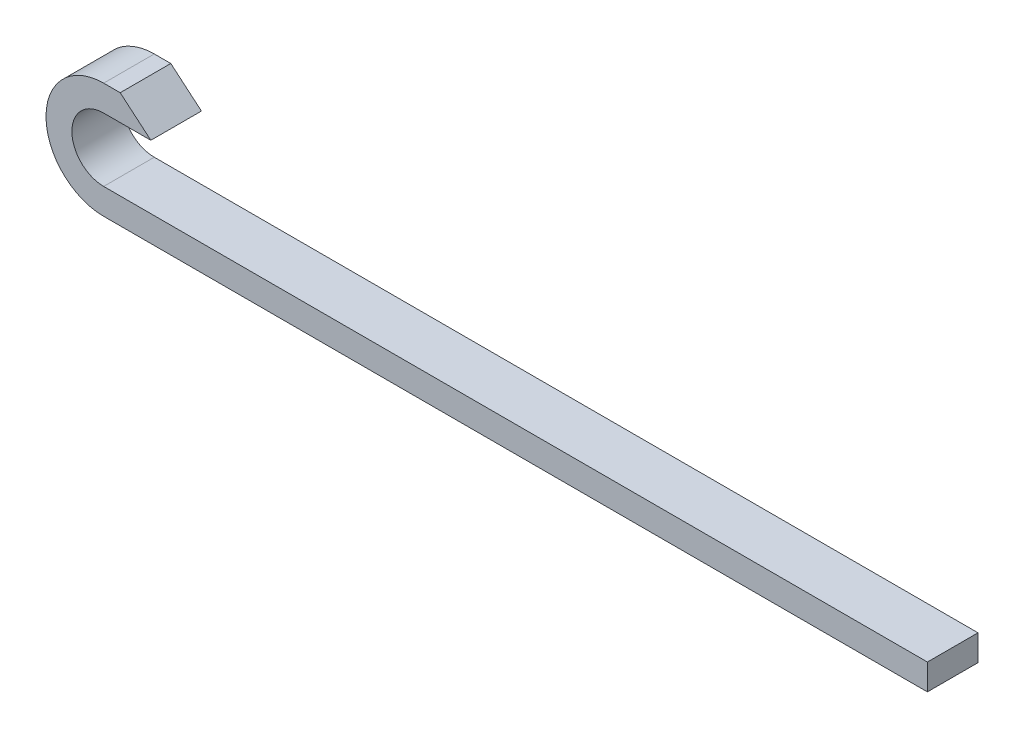
SolidWorks part; units mm, degrees
ref_plane "前视基准面" through (0, 0, 0) normal (0, 0, 1) x (1, 0, 0)
ref_plane "上视基准面" through (0, 0, 0) normal (0, 1, 0) x (1, 0, 0)
ref_plane "右视基准面" through (0, 0, 0) normal (1, 0, 0) x (0, 0, -1)
sketch "草图1" plane through (0, 0, 0) normal (0, 0, 1) x (1, 0, 0)
  line L1 (291.5789, -1) -> (-408.4211, -1)
  line L2 (291.5789, -1) -> (291.5789, 21)
  line L3 (291.5789, 21) -> (-408.4211, 21)
  line L5 (-357.8648, 97) -> (-315.3943, 75)
  line L7 (-408.4211, 97) -> (-357.8648, 97)
  line L8 (-408.4211, 75) -> (-315.3943, 75)
  arc A0 (-408.4211, -1) -> (-408.4211, 97) centre (-408.4211, 48) cw
  arc A1 (-408.4211, 75) -> (-408.4211, 21) centre (-408.4211, 48) ccw
  dimension "D1" = 700
  dimension "D2" = 22
  dimension "D3" = 98
extrude "凸台-拉伸1" add sketch "草图1" along normal blind 43
sketch "草图2" plane through (0, 0, 43) normal (0, 0, 1) x (1, 0, 0)
  line L0 (-394.3734, 97) -> (-368.3426, 75)
  line L1 (-357.8648, 97) -> (-408.4211, 97) construction
  line L2 (-394.3734, 160) -> (-394.3734, 43.98) construction
  line L3 (-408.4211, 75) -> (-315.3943, 75) construction
extrude "切除-拉伸1" cut sketch "草图2" against normal through all and the other way through all
